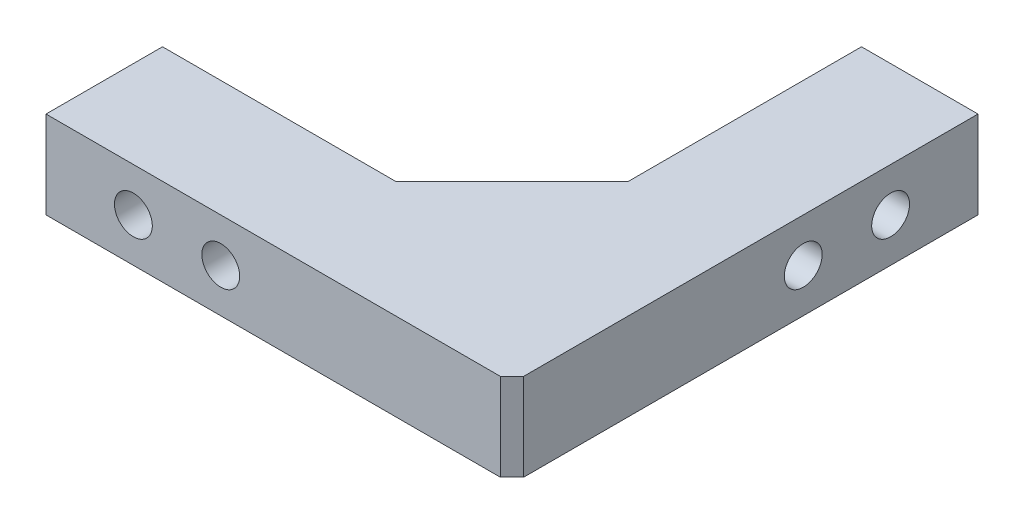
SolidWorks part; units mm, degrees
ref_plane "Front Plane" through (0, 0, 0) normal (0, 0, 1) x (1, 0, 0)
ref_plane "Top Plane" through (0, 0, 0) normal (0, 1, 0) x (1, 0, 0)
ref_plane "Right Plane" through (0, 0, 0) normal (1, 0, 0) x (0, 0, -1)
sketch "Sketch 3" plane through (0, 0, 0) normal (0, 1, 0) x (1, 0, 0)
  line L0 (40, 40) -> (20, 40)
  line L1 (-40, -40) -> (40, -40)
  line L2 (20, 40) -> (20, 0)
  line L3 (0, -20) -> (-40, -20)
  line L4 (40, -40) -> (40, 40)
  line L5 (-40, -40) -> (-40, -20)
  line L6 (20, 0) -> (0, -20)
  point P0 (0, 0)
  dimension "D1" = 20
  dimension "D2" = 80
  dimension "D3" = 20
  dimension "D4" = 80
  dimension "D5" = 40
  dimension "D6" = 40
extrude "Boss-Extrude 1" add sketch "Sketch 3" along normal blind 15
sketch "Sketch 4" plane through (0, 0, 20) normal (0, 0, -1) x (-1, 0, 0)
  line L0 (0, 15) -> (40, 15) construction
  circle A0 centre (10, 7.5) radius 3.25
  dimension "D1" = 6.5
  dimension "D2" = 7.5
  dimension "D3" = 50
extrude "Cut-Extrude 1" cut sketch "Sketch 4" against normal through all
pattern_linear "Linear Pattern 1" count 2 spacing 15 along (-1, 0, 0) of "Cut-Extrude 1"
sketch "Sketch 5" plane through (40, 0, 0) normal (1, 0, 0) x (0, 0, -1)
  line L0 (-40, 15) -> (-40, 0) construction
  line L1 (-40, 0) -> (40, 0) construction
  circle A0 centre (10, 7.5) radius 3.25
  dimension "D1" = 6.5
  dimension "D2" = 50
  dimension "D3" = 7.5
extrude "Cut-Extrude 2" cut sketch "Sketch 5" against normal through all
pattern_linear "Linear Pattern 2" count 2 spacing 15 along (0, 0, -1) of "Cut-Extrude 2"
chamfer "Chamfer 1" distance 2 angle 45 1 edges at (40, 7.5, 40)
